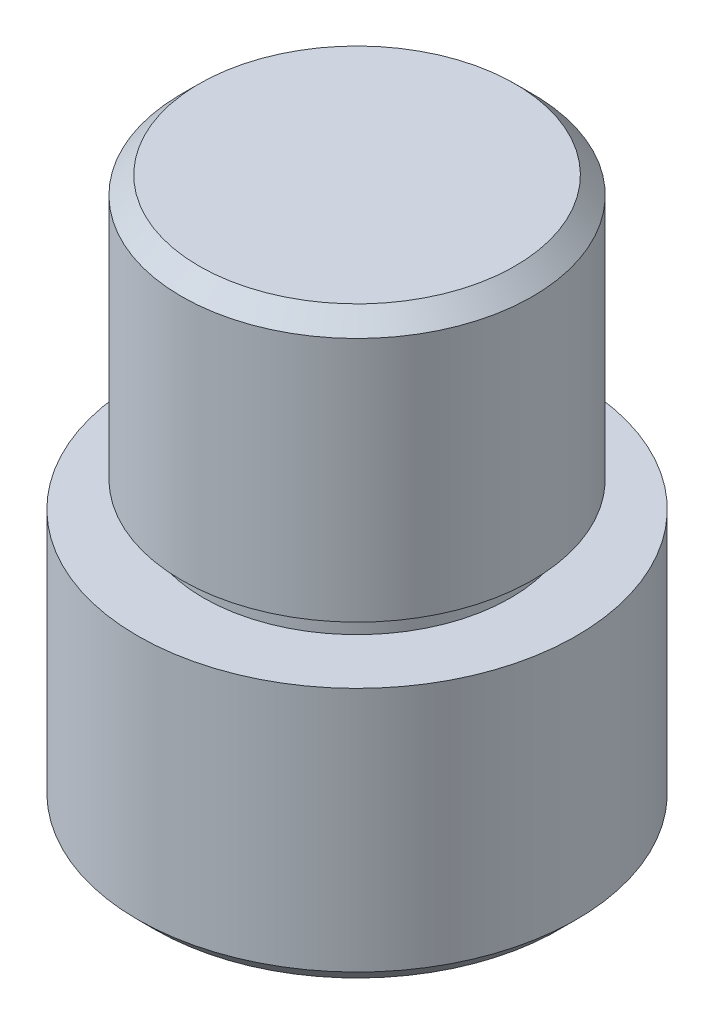
from build123d import *

# Parameters (mm, degrees)
SKETCH1_W     = 20
SKETCH1_H     = 30
SKETCH1_W_2   = 17.5
SKETCH1_H_2   = 3
CHAMFER1_SIZE = 2
CHAMFER2_SIZE = 2


with BuildPart() as part:
    # Sketch1 → Revolve1 (revolve)
    with BuildSketch(Plane.XY, mode=Mode.PRIVATE) as revolve1_sk:
        Polygon((0, -35.605263158), (0, -5.605263158), (-17.5, -5.605263158), (-25, -5.605263158), (-25, -35.605263158), align=None)
        with Locations((-10, 12.394736842)):
            Rectangle(SKETCH1_W, SKETCH1_H)
        with Locations((-8.75, -4.105263158)):
            Rectangle(SKETCH1_W_2, SKETCH1_H_2)
    revolve(revolve1_sk.sketch.rotate(Axis((0, 37.5, 0), (0, -1, 0)), 270), axis=Axis((0, 37.5, 0), (0, -1, 0)))

    # Chamfer1
    chamfer1_edges = [part.edges().sort_by_distance(p)[0] for p in [
        (0, 27.394736842, -20),
    ]]
    chamfer(chamfer1_edges, length=CHAMFER1_SIZE)

    # Chamfer2
    chamfer2_edges = [part.edges().sort_by_distance(p)[0] for p in [
        (0, -35.605263158, -25),
    ]]
    chamfer(chamfer2_edges, length=CHAMFER2_SIZE)


solid = part.part
